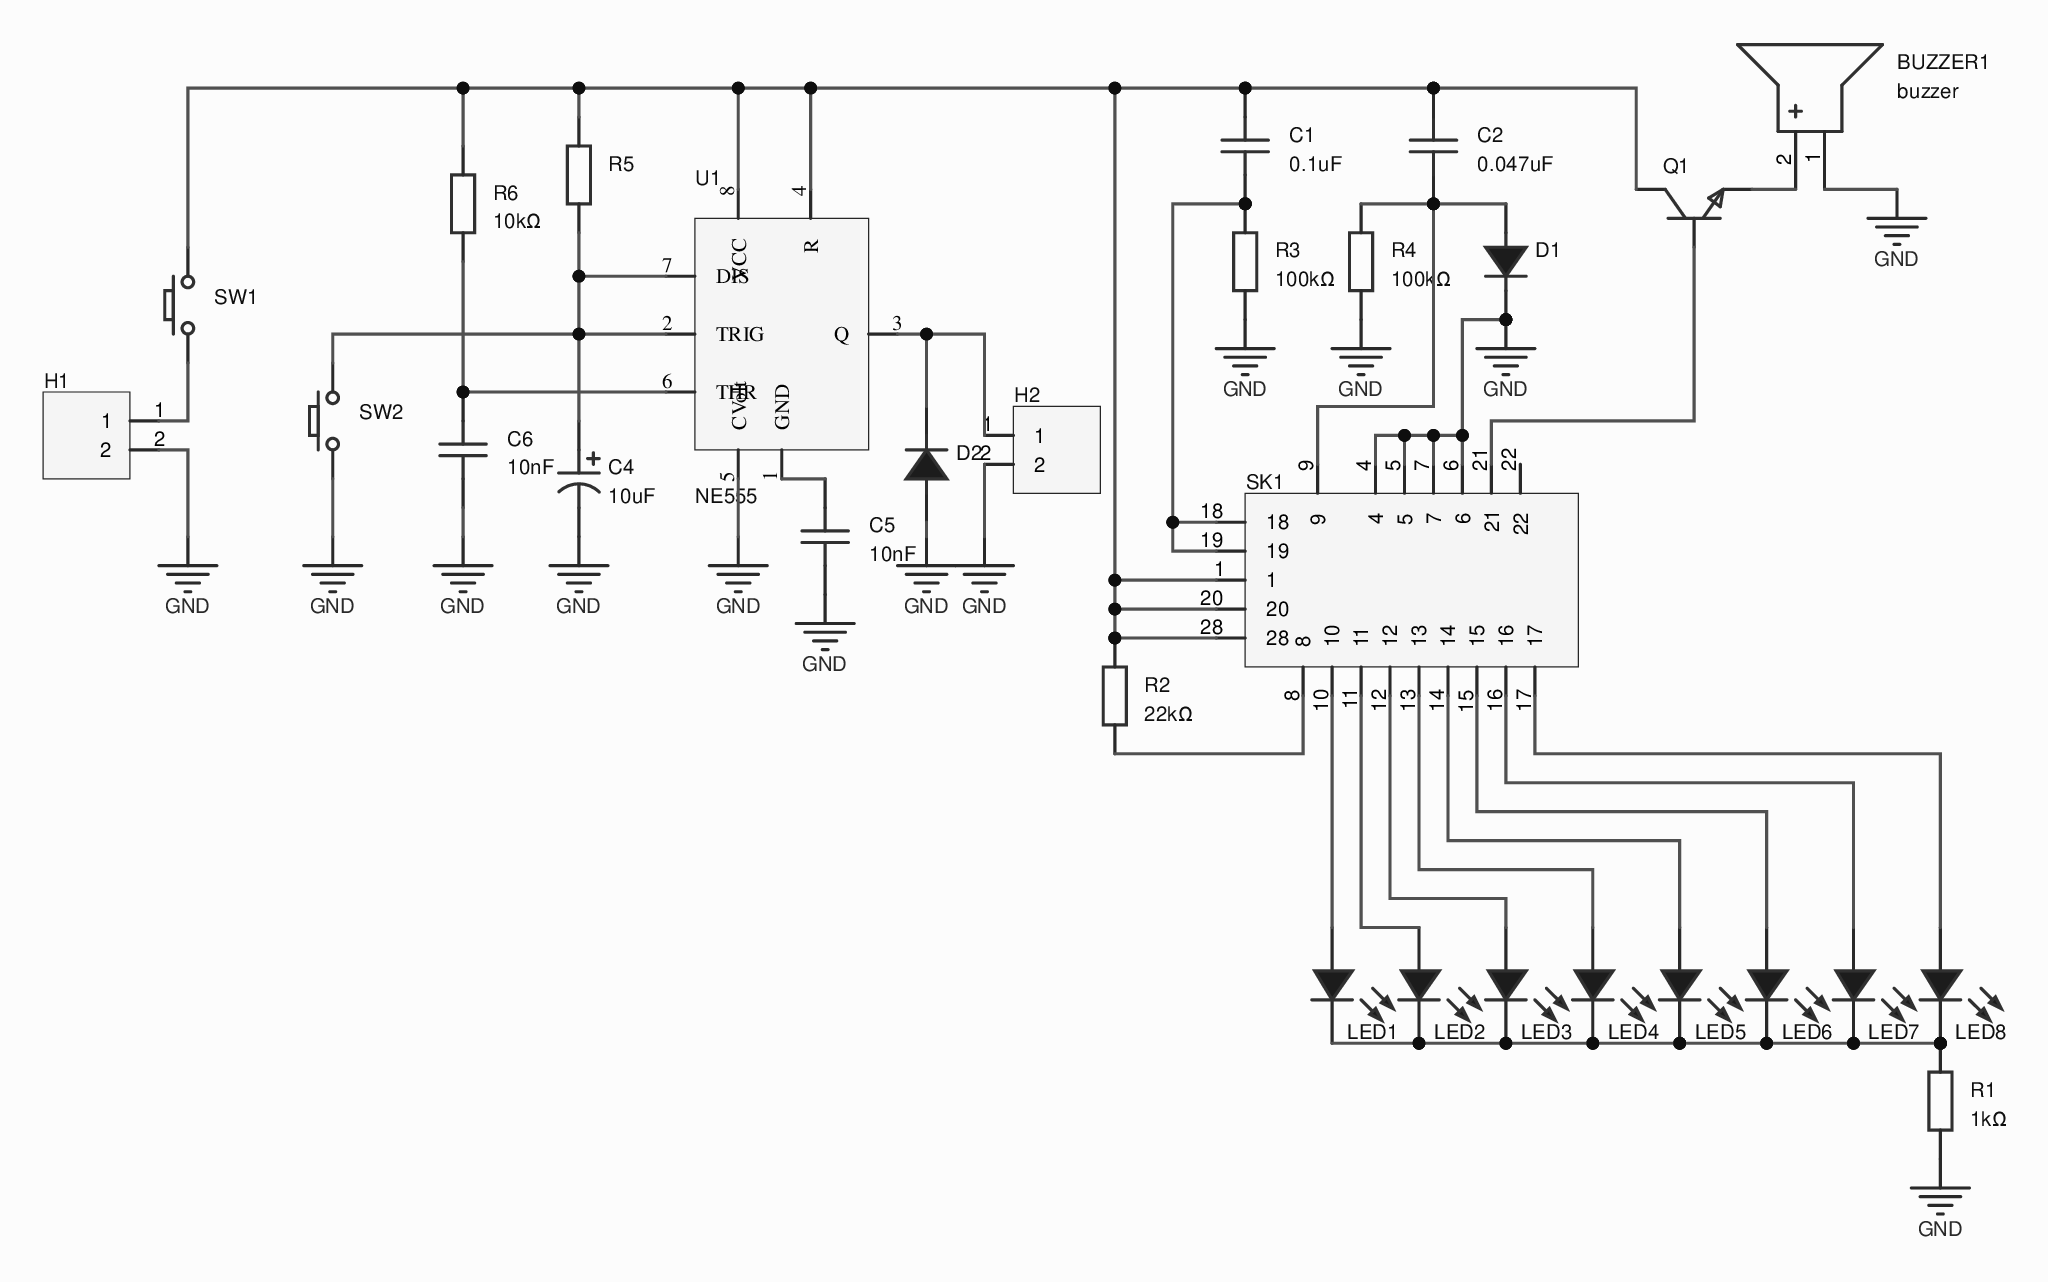
[diagram p0: MISC75112-3.schdoc]
# Altium project MISC75112-2.PrjPcb
1 sheet, 29 parts. Net scope: global (net labels, ports and power ports of the same name join across sheets).
Board file: MISC75112.pcbdoc

## Sheet MISC75112-3.schdoc
size 297 x 209 mm; Version: V1.0; @Project Name: MISC75112; @Update Date: 2026-09-24; @Create Date: 2026-09-24; @Board Name: MISC75112; @Create Time: 09:16:08; @Page Count: 1; @Page No: 1; @Schematic Name: MISC75112; @Update Time: 09:16:08; Size: A4

### Parts
BUZZER1  buzzer  [BUZ-TH_BD12.0-P6.00-D0.9-RD]
C1  0.1uF  [CAP-TH_L5.1-W3.2-P5.08-D0.50]
C2  0.047uF  [CAP-TH_L5.1-W3.2-P5.08-D0.50]
C4  10uF  [CAP-TH_BD5.0-P2.00-D0.8-FD-10UF50VC110GL]
C5  10nF  [CAP-TH_L5.1-W3.2-P5.08-D0.50]
C6  10nF  [CAP-TH_L5.1-W3.2-P5.08-D0.50]
D1  (no value)  [DO_1N4007]
D2  (no value)  [DO_1N4007]
H1  (no value)  [HDR-TH_2P-P2.54-V-M-1]
H2  (no value)  [HDR-TH_2P-P2.54-V-M-1]
LED1  (no value)  [LED-TH_5mm]
LED2  (no value)  [LED-TH_5mm]
LED3  (no value)  [LED-TH_5mm]
LED4  (no value)  [LED-TH_5mm]
LED5  (no value)  [LED-TH_5mm]
LED6  (no value)  [LED-TH_5mm]
LED7  (no value)  [LED-TH_5mm]
LED8  (no value)  [LED-TH_5mm]
Q1  (no value)  [S8050_TO_92]
R1  1kΩ  [Res_1/8W]
R2  22kΩ  [Res_1/8W]
R3  100kΩ  [Res_1/8W]
R4  100kΩ  [Res_1/8W]
R5  10kΩ  [Res_1/8W]  (value not drawn)
R6  10kΩ  [Res_1/8W]
SK1  X5621WV-2x14-C762D1000-1000  [DIP-28_L35.6-W10.2-P2.54-LS7.6-BL]  (value not drawn)
SW1  (no value)  [Key_TH_3.5x6x4.3]
SW2  (no value)  [Key_TH_3.5x6x4.3]
U1  NE555  [DIP-8_L9.8-W6.4-P2.54-LS7.6-BL]

### Nets
GND: BUZZER1.1(-) C4.2 C5.1 C6.1 D1.1(K) D2.2(A) H1.2 H2.2 R1.1 R3.1 R4.1 SK1.4 SK1.5 SK1.6 SK1.7 SW2.A U1.5(CVolt)
NetBUZZER1_2: BUZZER1.2(+) Q1.1(E)
NetC1_1: C1.1 R3.2 SK1.18 SK1.19
NetC1_2: C1.2 C2.2 Q1.3(C) R2.2 R5.2 R6.2 SK1.1 SK1.20 SK1.28 SW1.B U1.4(R) U1.8(VCC)
NetC2_1: C2.1 D1.2(A) R4.2 SK1.9
NetC4_1: C4.1 R5.1 SW2.B U1.2(TRIG) U1.7(DIS)
NetC5_2: C5.2 U1.1(GND)
NetC6_2: C6.2 R6.1 U1.6(THR)
NetD2_1: D2.1(K) H2.1 U1.3(Q)
NetH1_1: H1.1 SW1.A
NetLED1_1: LED1.1(C) SK1.10
NetLED1_2: LED1.2(A) LED2.2(A) LED3.2(A) LED4.2(A) LED5.2(A) LED6.2(A) LED7.2(A) LED8.2(A) R1.2
NetLED2_1: LED2.1(C) SK1.11
NetLED3_1: LED3.1(C) SK1.12
NetLED4_1: LED4.1(C) SK1.13
NetLED5_1: LED5.1(C) SK1.14
NetLED6_1: LED6.1(C) SK1.15
NetLED7_1: LED7.1(C) SK1.16
NetLED8_1: LED8.1(C) SK1.17
NetQ1_2: Q1.2(B) SK1.21
NetR2_1: R2.1 SK1.8

Not connected (* = marked no-connect by the designer): SK1 22

### Library data of the parts
BUZZER1 = buzzer: AddInBom: yes; ModelId: af17e4151ed84fc2a628230bf23763630819f05c4eef4c71ace90d822a990e87; ModelTransform: 472.44,472.176,0,270,0,0,0,0,-196.85; Symbol: BUZZER; Device: buzzer; FootprintName: BUZ-TH_BD12.0-P6.00-D0.9-RD; LCSC Part Name: buzzer; SupplierPart: C9900014030; ManufacturerPart: buzzer; Supplier Footprint: buzzer; JLCPCB Part Class: Extended Part; Supplier: LCSC; ConvertToPcb: yes; ModelName: BUZ-TH_BD12.0-P6.00-D0.9-RD
C1 C2 C5 C6 = C323C104K5R5TA7301: 容值:100nF;精度:±10%;额定电压:50V;温度系数:X7R;; Manufacturer: KEMET(基美); AddInBom: yes; ModelId: 5e578892460b443ea6286c5f4e214fbb0819f05c4eef4c71ace90d822a990e87; ModelTransform: 219.6846,125.5903,0,0,0,0,0,0,-196.85; Tolerance: ±10%; Voltage Rating: 50V; Temperature Coefficient: X7R; Pin Spacing: 5.08mm; Symbol: C323C104K5R5TA7301; Device: C323C104K5R5TA7301; FootprintName: CAP-TH_L5.1-W3.2-P5.08-D0.50; LCSC Part Name: 100nF ±10% 50V; ManufacturerPart: C323C104K5R5TA7301; Supplier Footprint: 插件,P=5.08mm; JLCPCB Part Class: Extended Part; Datasheet: https://item.szlcsc.com/datasheet/C323C104K5R5TA7301/194969.html; Supplier: LCSC; ConvertToPcb: yes; ModelName: CAP-TH_L5.1-W3.2-P5.08-D0.50
  C1: Value: 0.1uF
  C2: Value: 0.047uF
  C5 C6: Value: 10nF
C4 = 10UF50VC110GL: 容值:10uF;精度:±20%;额定电压:50V;纹波电流:120mA@100KHz;等效串联电阻(ESR):1.6Ω;; Manufacturer: Econd(米朗电子); 3D Model: b35ab6b0460c4c43a629d91cfc2b58780819f05c4eef4c71ace90d822a990e87; 3D Model Transform: 196.85,196.85,0,0,0,0,0,0,-196.85; Tolerance: ±20%; Voltage Rating: 50V; Equivalent Series Resistance(ESR): 1.6Ω; Pin Spacing: 2mm; Lifetime: 5000hrs@105℃; AddInBom: yes; Symbol: 10UF50VC110GL; Device: 10UF50VC110GL; LCSC Part Name: 10uF ±20% 50V; Supplier Part: C46867109; Manufacturer Part: 10UF50VC110GL; Supplier Footprint: 插件,D5xL11mm; JLCPCB Part Class: Extended Part; Datasheet: https://item.szlcsc.com/datasheet/10UF50VC110GL/49031974.html; Supplier: LCSC; Value: 10uF; Ripple Current: 120mA@100KHz; Diameter: 5mm; Height - Seated (Max): 11mm; Operating Temperature: -40℃~+105℃; FootprintName: CAP-TH_BD5.0-P2.00-D0.8-FD-10UF50VC110GL; ConvertToPcb: yes; ModelName: CAP-TH_BD5.0-P2.00-D0.8-FD-10UF50VC110GL
D1 D2 = D_1N4007A: AddInBom: yes; ModelId: 6de1e9b71a0d4751b4e9df530304c1a30819f05c4eef4c71ace90d822a990e87; ModelName: DO-41_D2.4-L4.7-P8.70; ModelTransform: 373.9,94.4,232.29,0,0,0,0,0,-140; Symbol: D_1N4007; Device: D_1N4007A; FootprintName: DO_1N4007; Supplier Footprint: DO-41; ConvertToPcb: yes
H1 H2 = HDR-M_2.54_1x2P: Symbol: 210S-1*2P L=11.6MMGold-plated black; 3D Model: 79b2e9f2d70a4d68a1b7098f27c6d4c50819f05c4eef4c71ace90d822a990e87; 3D Model Transform: 200,100,0,0,0,0,0,0,-118.11; ConvertToPcb: yes; ModelName: HDR-M-2.54_1x2; Device: HDR-M_2.54_1x2P; Supplier Part: C124375; Supplier Footprint: 插件; FootprintName: HDR-TH_2P-P2.54-V-M-1; AddInBom: yes
LED1-LED8 = LED_TH-B_5mm: AddInBom: yes; ModelId: b0e300213b7e4bc9906214592eb37e0a0819f05c4eef4c71ace90d822a990e87; ModelName: LED-TH_BD5.0_Blue; ModelTransform: 177.89258,177.84487,480.30997,90,0,0,-1.9685,0,-389.76378; Symbol: LED_TH-B; Device: LED_TH-B_5mm; FootprintName: LED-TH_5mm; ConvertToPcb: yes; Supplier Footprint: 插件
Q1 = S8050_TO_NPN: ConvertToPcb: yes; ModelId: aafe8e06f2154e7c93506efd0d6632dd0819f05c4eef4c71ace90d822a990e87; ModelName: TO-92-3_L4.9-W3.7-P1.27-L; ModelTransform: 180.78,141.44,417.3,0,0,0,0,0,-200; Symbol: S8050_TO_NPN; Device: S8050_TO_NPN; FootprintName: S8050_TO_92; AddInBom: yes; Supplier Footprint: TO-92
R1-R6 = Res_AXIAL-1/8W: Symbol: Resistor; 3D Model: b2b5ae7ae4c642178fe0039925c86a3f0819f05c4eef4c71ace90d822a990e87; 3D Model Transform: 282.86,66.88,253.09,0,0,0,0,0,-191; ConvertToPcb: yes; ModelName: RES-TH_BD1.8-L3.2-P7.20-D0.4; Device: Res_AXIAL-1/8W; Supplier Footprint: 轴向引线; FootprintName: Res_1/8W; AddInBom: yes
  R1: Value: 1kΩ
  R2: Value: 22kΩ
  R3 R4: Value: 100kΩ
  R5 R6: Value: 10kΩ
SK1 = X5621WV-2x14-C762D1000-1000: 适配封装类型:DIP;间距:2.54mm;行距:7.62mm;圆孔/方孔:圆孔;总PIN数:28P;工作温度:-40℃~+105℃;; Manufacturer: XKB Connection(中国星坤); AddInBom: yes; ModelId: c649a9c93f8a44a2908aac05ade01b3f0819f05c4eef4c71ace90d822a990e87; ModelTransform: 1399.997,398.0307,0,180,0,0,0,0,-157.48; Adaptation Package Type: DIP; Pitch: 2.54mm; Row Spacing: 7.62mm; Circular Holes/Square Holes: Round hole; Number of Positions: 28P; Symbol: X5621WV-2X14-C762D1000-1000; Device: X5621WV-2x14-C762D1000-1000; FootprintName: DIP-28_L35.6-W10.2-P2.54-LS7.6-BL; LCSC Part Name: 间距2.54mm P数:28P 圆孔; SupplierPart: C2883639; ManufacturerPart: X5621WV-2x14-C762D1000-1000; Supplier Footprint: DIP-28; JLCPCB Part Class: Extended Part; Datasheet: https://item.szlcsc.com/datasheet/X5621WV-2x14-C762D1000-1000/3094131.html; Supplier: LCSC; ConvertToPcb: yes; ModelName: DIP-28_L35.6-W10.2-P2.54-LS7.6-BL; Operating Temperature: -40℃~+105℃
SW1 SW2 = Key_TH_3.5x6x4.3: ConvertToPcb: yes; ModelId: c3523f9014d949d7ba5445190a3178990819f05c4eef4c71ace90d822a990e87; ModelName: SW-TH_L6.0-W3.5-H5.0-P6.5; ModelTransform: 308.49,137.8,335.08,0,0,0,0,0,-129.92; Symbol: Key_TH_3.5x6x4.3; Device: Key_TH_3.5x6x4.3; FootprintName: Key_TH_3.5x6x4.3; AddInBom: yes; Supplier Footprint: 插件
U1 = NE555: Manufacturer: TI; ManufacturerPart: NE555DR; AddInBom: yes; Pin Type: IN; OriginFootprint: SOIC-8_L4.9-W3.9-P1.27-LS6.0-BL; Symbol: NE555; Device: NE555; FootprintName: DIP-8_L9.8-W6.4-P2.54-LS7.6-BL; ConvertToPcb: yes; Supplier: LCSC; image: C7593.jpg; SupplierPart: C7593; JLCPCB Part Class: Basic; NO_CONNECT: yes